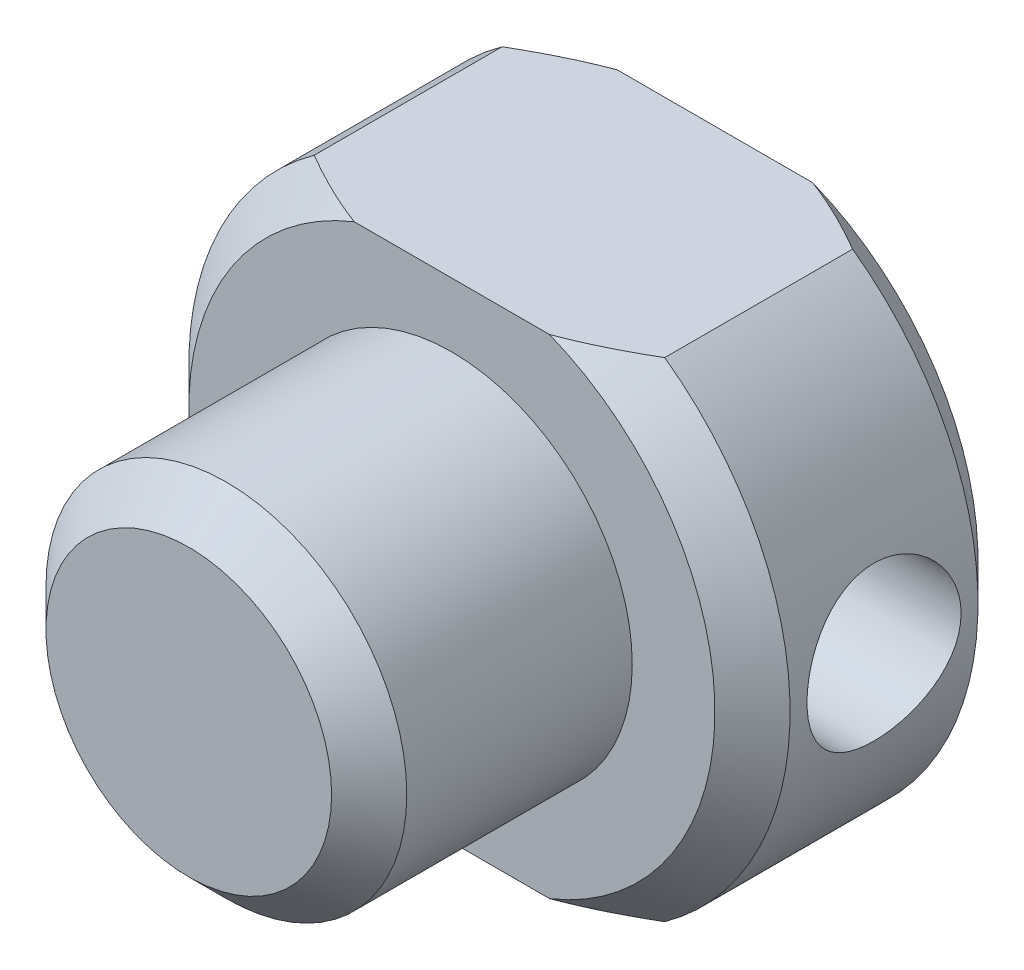
from build123d import *

# Parameters (mm, degrees)
SKETCH1_R                = 4
BOSS_EXTRUDE1_DEPTH      = 3.5
SKETCH3_R                = 2.4
BOSS_EXTRUDE2_DEPTH      = 3.5
SKETCH2_R                = 1.5
CUT_EXTRUDE1_DEPTH       = 6
M2_5_TAPPED_HOLE1_REACH  = 13.358
M2_5_TAPPED_HOLE1_BORE_R = 1.025
CHAMFER1_SIZE            = 0.5
SKETCH6_OUTSIDE_W        = 12.66
SKETCH6_OUTSIDE_H        = 12.66
SKETCH6_OUTSIDE_W_2      = 11.194211724
SKETCH6_OUTSIDE_H_2      = 6.5
CUT_EXTRUDE2_DEPTH       = 10


with BuildPart() as part:
    # Sketch1 → Boss-Extrude1 (new body)
    with BuildSketch(Plane.XY):
        Circle(SKETCH1_R)
    extrude(amount=BOSS_EXTRUDE1_DEPTH)

    # Sketch3 → Boss-Extrude2 (add)
    with BuildSketch(Plane.XY.offset(3.5)):
        Circle(SKETCH3_R)
    extrude(amount=BOSS_EXTRUDE2_DEPTH)

    # Sketch2 → Cut-Extrude1 (cut)
    with BuildSketch(Plane(origin=(0, 0, 0), x_dir=(-1, 0, 0), z_dir=(0, 0, -1))):
        Circle(SKETCH2_R)
    extrude(amount=-CUT_EXTRUDE1_DEPTH, mode=Mode.SUBTRACT)

    # M2.5 Tapped Hole1 bore → M2.5 Tapped Hole1 (cut, up to next)
    with BuildSketch(Plane(origin=(4, 0, 0), x_dir=(0, 0, -1), z_dir=(1, 0, 0)), mode=Mode.PRIVATE) as m2_5_tapped_hole1_sk1:
        with Locations((-1.75, 0)):
            Circle(M2_5_TAPPED_HOLE1_BORE_R)
    m2_5_tapped_hole1_tool1 = extrude(m2_5_tapped_hole1_sk1.sketch, amount=-M2_5_TAPPED_HOLE1_REACH, mode=Mode.PRIVATE) & part.part
    add(m2_5_tapped_hole1_tool1.solids().sort_by_distance((4, 0, 1.75))[0], mode=Mode.SUBTRACT)

    # Chamfer1
    chamfer1_edges = [part.edges().sort_by_distance(p)[0] for p in [
        (-4, 0, 0),
        (-4, 0, 3.5),
        (-2.4, 0, 7),
    ]]
    chamfer(chamfer1_edges, length=CHAMFER1_SIZE)

    # Sketch6 outside → Cut-Extrude2 (cut)
    with BuildSketch(Plane.XY.offset(3.5)):
        Rectangle(SKETCH6_OUTSIDE_W, SKETCH6_OUTSIDE_H)
        Rectangle(SKETCH6_OUTSIDE_W_2, SKETCH6_OUTSIDE_H_2, mode=Mode.SUBTRACT)
    extrude(amount=-CUT_EXTRUDE2_DEPTH, mode=Mode.SUBTRACT)


solid = part.part
